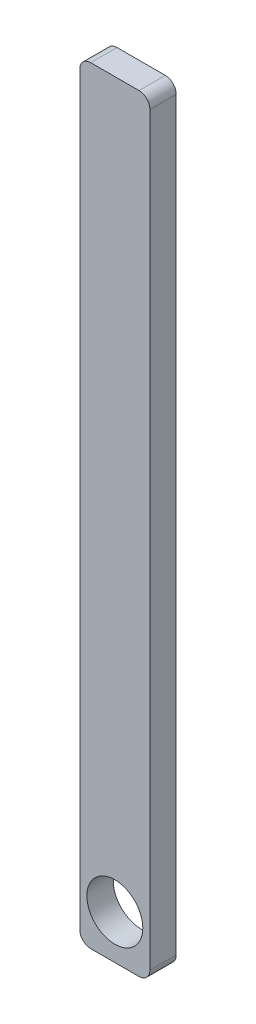
from build123d import *

# Parameters (mm, degrees)
SKETCH1_R           = 12.75
BOSS_EXTRUDE1_DEPTH = 12


with BuildPart() as part:
    # Sketch1 → Boss-Extrude1 (new body)
    with BuildSketch(Plane.XY):
        with BuildLine():
            Line((5, 0), (27, 0))
            ThreePointArc((27, 0), (30.535533906, 1.464466094), (32, 5))
            Line((32, 5), (32, 345))
            ThreePointArc((32, 345), (30.535533906, 348.535533906), (27, 350))
            Line((27, 350), (5, 350))
            ThreePointArc((5, 350), (1.464466094, 348.535533906), (0, 345))
            Line((0, 345), (0, 5))
            ThreePointArc((0, 5), (1.464466094, 1.464466094), (5, 0))
        make_face()
        with Locations((16, 20)):
            Circle(SKETCH1_R, mode=Mode.SUBTRACT)
    extrude(amount=BOSS_EXTRUDE1_DEPTH)


solid = part.part
